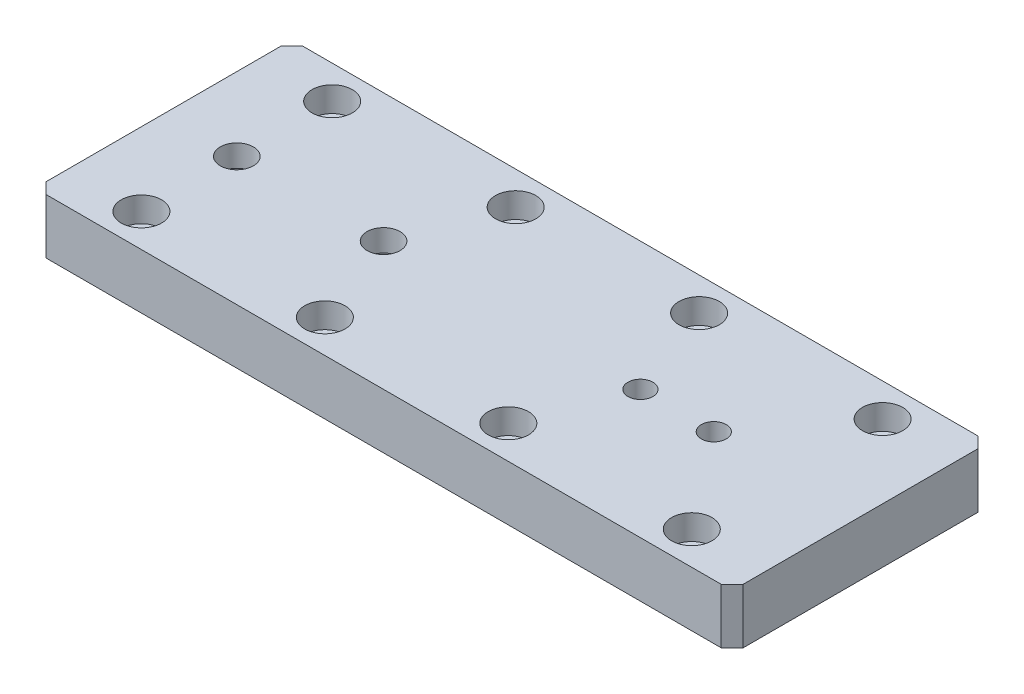
SolidWorks part; units mm, degrees
material "A6061"
ref_plane "前基準面" through (0, 0, 0) normal (0, 0, 1) x (1, 0, 0)
ref_plane "上基準面" through (0, 0, 0) normal (0, 1, 0) x (1, 0, 0)
ref_plane "右基準面" through (0, 0, 0) normal (1, 0, 0) x (0, 0, -1)
sketch "草图1" plane through (0, 0, 0) normal (0, 1, 0) x (1, 0, 0)
  line L1 (-95, 35) -> (95, 35)
  line L2 (-95, 35) -> (-95, -35)
  line L3 (-95, -35) -> (95, -35)
  line L4 (95, 35) -> (95, -35)
  line L5 (-95, 35) -> (95, -35) construction
  line L6 (-95, -35) -> (95, 35) construction
  point P0 (0, 0)
  dimension "D1" = 70
  dimension "D2" = 190
extrude "凸台-拉伸1" add sketch "草图1" along normal blind 15
chamfer "倒角1" distance 3 angle 45 4 edges at (-95, 7.5, -35) (-95, 7.5, 35) (95, 7.5, -35) (95, 7.5, 35)
hole_wizard "打孔尺寸(%根据)内六角圆柱头螺钉的类型5" positions "草图2" profile "草图3" counterbore size "M6" standard "GB" end condition through all
sketch "草图2" plane through (0, 15, 0) normal (0, 1, 0) x (1, 0, 0)
  line L0 (0, 0) -> (202.3318, 0) construction
  line L2 (95, -32) -> (95, 32) construction
  point P0 (75, -26)
  point P12 (25, -26)
  point P13 (-25, -26)
  point P14 (-75, -26)
  point P15 (25, 26)
  point P16 (-25, 26)
  point P17 (-75, 26)
  point P18 (75, 26)
  dimension "D1" = 4
  dimension "D3" = 20
  dimension "D4" = 52
  dimension "D5" = 50
  dimension "D2" = 2
sketch "草图3" plane through (75, 15, 26) normal (1, 0, 0) x (0, 0, 1)
  line L0 (0, 0) -> (0, 15)
  line L1 (0, 15) -> (3.3, 15)
  line L3 (3.3, 15) -> (3.3, 6.8)
  line L4 (3.3, 6.8) -> (5.5, 6.8)
  line L5 (5.5, 6.8) -> (5.5, 0)
  line L7 (5.5, 0) -> (0, 0)
  line L11 (0, -6.35) -> (0, 107.95) construction
  dimension "通孔孔直径" = 6.6
  dimension "通孔孔深度" = 15
  dimension "柱形沉头孔直径" = 11
  dimension "柱形沉头孔深度" = 6.8
hole_wizard "打孔尺寸(%根据)内六角圆柱头螺钉的类型3" positions "草图4" profile "草图5" counterbore size "M8" standard "GB" end condition through all
sketch "草图4" plane through (0, 0, 0) normal (0, -1, 0) x (-1, 0, 0)
  line L0 (0, 0) -> (0, -83.5862) construction
  line L1 (95, 32) -> (95, -32) construction
  line L3 (0, 0) -> (147.517, 0) construction
  point P0 (35, 0)
  point P5 (75, 0)
  dimension "D2" = 40
  dimension "D3" = 20
sketch "草图5" plane through (-35, 0, 0) normal (1, 0, 0) x (0, 0, -1)
  line L0 (0, 0) -> (0, 15)
  line L1 (0, 15) -> (4.5, 15)
  line L3 (4.5, 15) -> (4.5, 9)
  line L4 (4.5, 9) -> (7.5, 9)
  line L5 (7.5, 9) -> (7.5, 0)
  line L7 (7.5, 0) -> (0, 0)
  line L11 (0, -6.35) -> (0, 107.95) construction
  dimension "通孔孔直径" = 9
  dimension "通孔孔深度" = 15
  dimension "柱形沉头孔直径" = 15
  dimension "柱形沉头孔深度" = 9
hole_wizard "M6 螺纹孔2" positions "草图8" profile "草图9" tap size "M6" standard "GB"
sketch "草图8" plane through (0, 15, 0) normal (0, 1, 0) x (1, 0, 0)
  line L0 (0, 0) -> (-88.3626, 0) construction
  line L2 (-95, 32) -> (-95, -32) construction
  point P0 (5, -21)
  point P2 (55, -21)
  point P9 (55, 21)
  point P10 (5, 21)
  dimension "D1" = 42
  dimension "D2" = 50
  dimension "D3" = 100
sketch "草图9" plane through (5, 15, 21) normal (1, 0, 0) x (0, 0, 1)
  line L0 (0, 0) -> (0, 15)
  line L1 (0, 15) -> (2.5, 15)
  line L2 (2.5, 15) -> (2.5, 0)
  line L5 (2.5, 0) -> (0, 0)
  line L11 (0, -6.35) -> (0, 107.95) construction
  dimension "通孔螺纹孔钻头直径" = 5
  dimension "通孔螺纹孔钻头深度" = 15
cosmetic thread "孔螺蚊线3" [suppressed] parameters "D2"=6
cosmetic thread "孔螺蚊线4" [suppressed] parameters "D2"=6
cosmetic thread "孔螺蚊线5" [suppressed] parameters "D2"=6
cosmetic thread "孔螺蚊线6" [suppressed] parameters "D2"=6
hole_wizard "M8 螺纹孔1" positions "草图10" profile "草图11" tap size "M8" standard "GB" end condition through all
sketch "草图10" plane through (0, 15, 0) normal (0, 1, 0) x (1, 0, 0)
  line L0 (95, -32) -> (95, 32) construction
  point P0 (55, 0)
  point P2 (35, 0)
  dimension "D1" = 20
  dimension "D2" = 40
sketch "草图11" plane through (55, 15, 0) normal (1, 0, 0) x (0, 0, 1)
  line L0 (0, 0) -> (0, 15)
  line L1 (0, 15) -> (3.4, 15)
  line L2 (3.4, 15) -> (3.4, 0)
  line L5 (3.4, 0) -> (0, 0)
  line L11 (0, -6.35) -> (0, 107.95) construction
  dimension "通孔螺纹孔钻头直径" = 6.8
  dimension "通孔螺纹孔钻头深度" = 15
cosmetic thread "孔螺蚊线7" parameters "D2"=8
cosmetic thread "孔螺蚊线8" parameters "D2"=8
